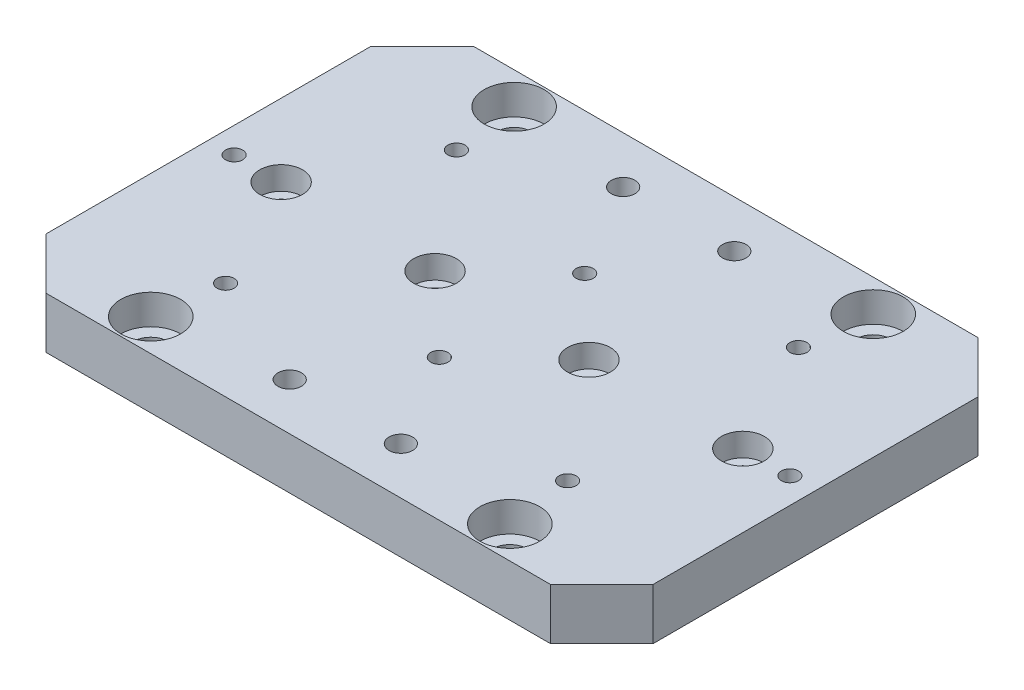
from build123d import *

# Parameters (mm, degrees)
SKETCH1_W                                           = 142
SKETCH1_H                                           = 100
EXTRUDE1_DEPTH                                      = 12
CBORE_FOR_M5_HEX_SOCKET_HEAD_CAP_SCREW1_D           = 5.5
CBORE_FOR_M5_HEX_SOCKET_HEAD_CAP_SCREW1_CBORE_D     = 10
CBORE_FOR_M5_HEX_SOCKET_HEAD_CAP_SCREW1_CBORE_DEPTH = 5.4
CBORE_FOR_M5_HEX_SOCKET_HEAD_CAP_SCREW2_D           = 5.5
CBORE_FOR_M5_HEX_SOCKET_HEAD_CAP_SCREW2_CBORE_D     = 10
CBORE_FOR_M5_HEX_SOCKET_HEAD_CAP_SCREW2_CBORE_DEPTH = 5.4
MM_0_D                                              = 4
CHAMFER1_SIZE                                       = 12
F_4_0_MM_DOWEL_HOLES1_D                             = 4
F_8_0_MM_DOWEL_HOLES1_D                             = 8
SKETCH13_R                                          = 7
EXTRUDE2_DEPTH                                      = 7
F_4_0_MM_DOWEL_HOLES2_D                             = 4


with BuildPart() as part:
    # Sketch1 → Extrude1 (new body)
    with BuildSketch(Plane(origin=(0, 0, 0), x_dir=(1, 0, 0), z_dir=(0, 1, 0))):
        Rectangle(SKETCH1_W, SKETCH1_H)
    extrude(amount=EXTRUDE1_DEPTH)

    # CBORE for M5 Hex Socket Head Cap Screw1 (through all)
    with Locations(Plane(origin=(0, 0, 0), x_dir=(-1, 0, 0), z_dir=(0, -1, 0))):
        with Locations((-13, -39), (13, 39), (-13, 39), (13, -39)):
            CounterBoreHole(CBORE_FOR_M5_HEX_SOCKET_HEAD_CAP_SCREW1_D / 2, CBORE_FOR_M5_HEX_SOCKET_HEAD_CAP_SCREW1_CBORE_D / 2, CBORE_FOR_M5_HEX_SOCKET_HEAD_CAP_SCREW1_CBORE_DEPTH)

    # CBORE for M5 Hex Socket Head Cap Screw2 (through all)
    with Locations(Plane(origin=(0, 12, 0), x_dir=(1, 0, 0), z_dir=(0, 1, 0))):
        with Locations((-54, 0), (54, 0), (-18, 0), (18, 0)):
            CounterBoreHole(CBORE_FOR_M5_HEX_SOCKET_HEAD_CAP_SCREW2_D / 2, CBORE_FOR_M5_HEX_SOCKET_HEAD_CAP_SCREW2_CBORE_D / 2, CBORE_FOR_M5_HEX_SOCKET_HEAD_CAP_SCREW2_CBORE_DEPTH)

    # 大小mm 暗销孔0 (through all)
    with Locations(Plane(origin=(0, 12, 0), x_dir=(1, 0, 0), z_dir=(0, 1, 0))):
        with Locations((-40, 27), (40, 27), (40, -27), (-40, -27)):
            Hole(MM_0_D / 2)

    # Chamfer1
    chamfer1_edges = [part.edges().sort_by_distance(p)[0] for p in [
        (-71, 6, -50),
        (71, 6, -50),
        (71, 6, 50),
        (-71, 6, 50),
    ]]
    chamfer(chamfer1_edges, length=CHAMFER1_SIZE)

    # Ø4.0 mm Dowel Holes1 (through all)
    with Locations(Plane(origin=(0, 12, 0), x_dir=(1, 0, 0), z_dir=(0, 1, 0))):
        with Locations((-65, 0), (65, 0)):
            Hole(F_4_0_MM_DOWEL_HOLES1_D / 2)

    # Ø8.0 mm Dowel Holes1 (through all)
    with Locations(Plane(origin=(0, 12, 0), x_dir=(1, 0, 0), z_dir=(0, 1, 0))):
        with Locations((-42, 42.5), (42, 42.5), (42, -42.5), (-42, -42.5)):
            Hole(F_8_0_MM_DOWEL_HOLES1_D / 2)

    # Sketch13 → Extrude2 (cut)
    with BuildSketch(Plane(origin=(0, 12, 0), x_dir=(1, 0, 0), z_dir=(0, 1, 0))):
        with Locations(Location((-42, -42.5, 0), (0, 0, 270))):
            Circle(SKETCH13_R)
        with Locations(Location((42, -42.5, 0), (0, 0, 270))):
            Circle(SKETCH13_R)
        with Locations(Location((-42, 42.5, 0), (0, 0, 270))):
            Circle(SKETCH13_R)
        with Locations(Location((42, 42.5, 0), (0, 0, 270))):
            Circle(SKETCH13_R)
    extrude(amount=-EXTRUDE2_DEPTH, mode=Mode.SUBTRACT)

    # Ø4.0 mm Dowel Holes2 (through all)
    with Locations(Plane(origin=(0, 0, 0), x_dir=(-1, 0, 0), z_dir=(0, -1, 0))):
        with Locations((0, 17), (0, -17)):
            Hole(F_4_0_MM_DOWEL_HOLES2_D / 2)


solid = part.part
